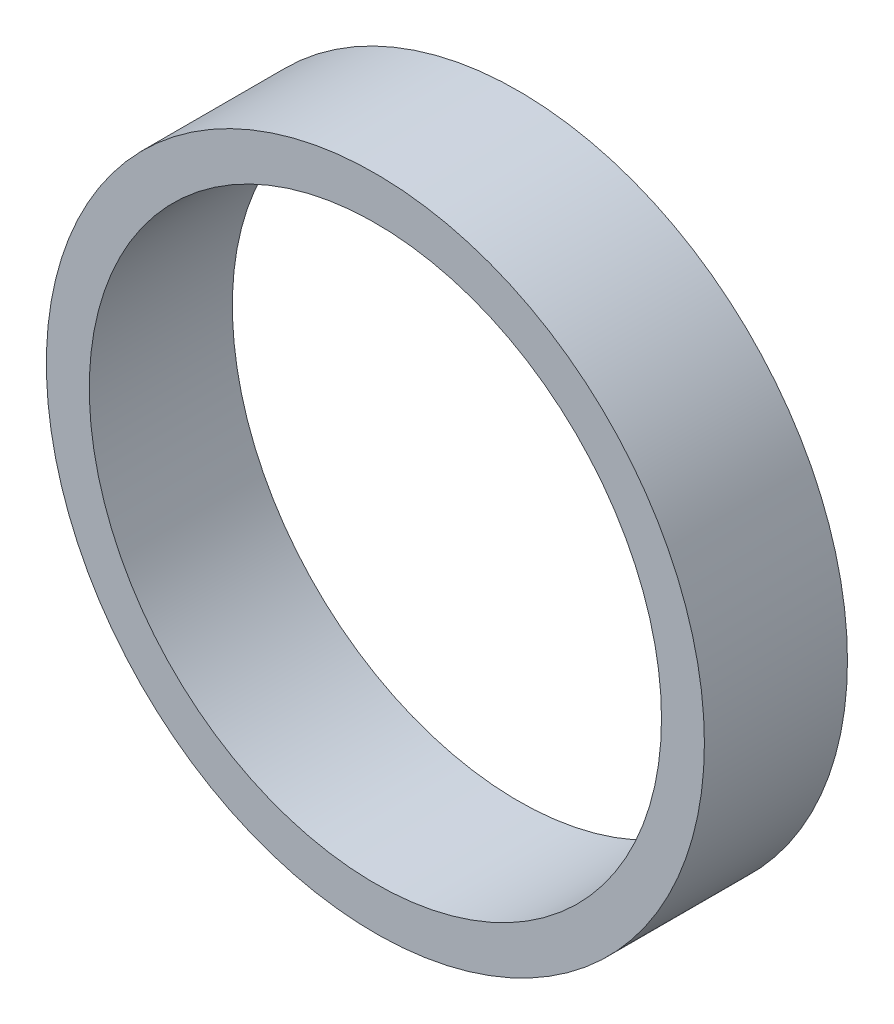
SolidWorks part; units mm, degrees
ref_plane "Front Plane" through (0, 0, 0) normal (0, 0, 1) x (1, 0, 0)
ref_plane "Top Plane" through (0, 0, 0) normal (0, 1, 0) x (1, 0, 0)
ref_plane "Right Plane" through (0, 0, 0) normal (1, 0, 0) x (0, 0, -1)
sketch "Sketch1" plane through (0, 0, 0) normal (0, 0, 1) x (1, 0, 0)
  circle A0 centre (0, 0) radius 115
  circle A1 centre (0, 0) radius 100
  dimension "D1" = 230
  dimension "D2" = 200
extrude "Boss-Extrude1" add sketch "Sketch1" along normal mid plane 50
